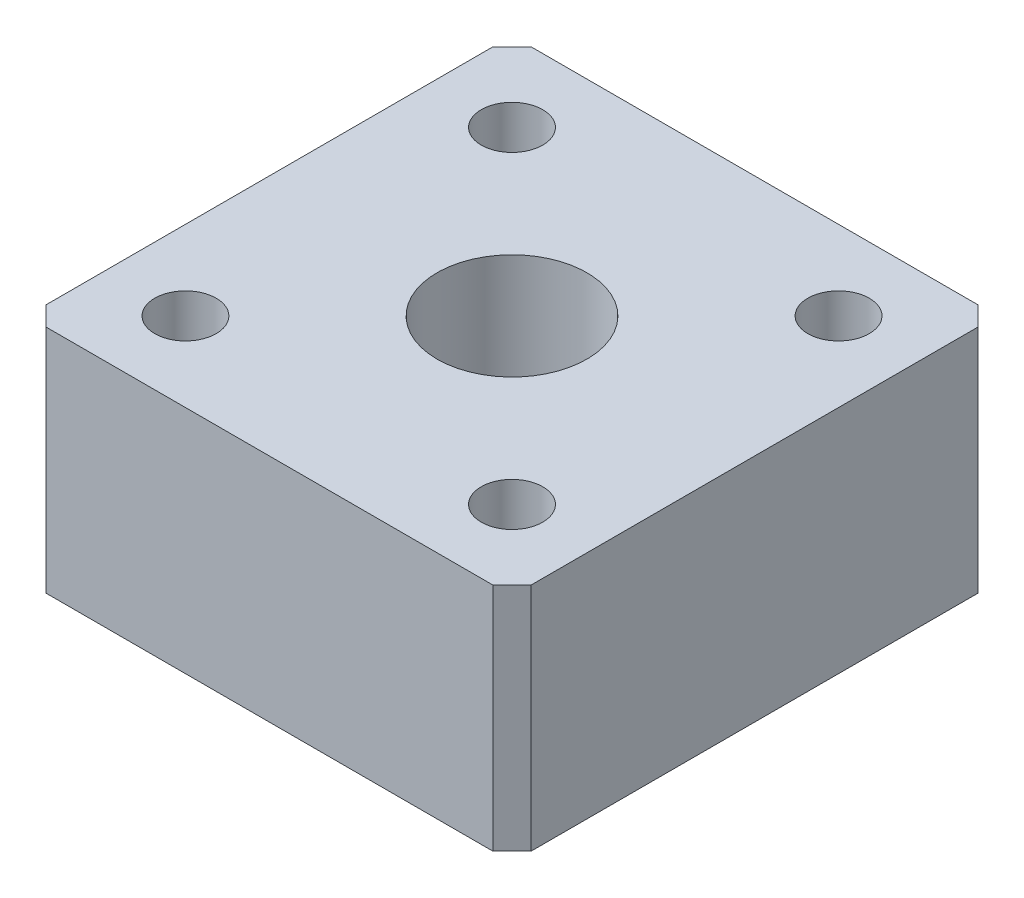
from build123d import *

# Parameters (mm, degrees)
SKETCH1_R             = 1.95
BOSS_EXTRUDE1_DEPTH   = 6
M2_TAPPED_HOLE2_D     = 1.6
M2_TAPPED_HOLE2_DEPTH = 6
M2_TAPPED_HOLE2_TIP   = 572.957422794


with BuildPart() as part:
    # Sketch1 → Boss-Extrude1 (new body)
    with BuildSketch(Plane(origin=(0, 0, 0), x_dir=(1, 0, 0), z_dir=(0, 1, 0))):
        Polygon((-6.315, 5.815), (-5.815, 6.315), (5.815, 6.315), (6.315, 5.815), (6.315, -5.815), (5.815, -6.315), (-5.815, -6.315), (-6.315, -5.815), align=None)
        with Locations(Location((0, 0, 0), (0, 0, 270))):
            Circle(SKETCH1_R, mode=Mode.SUBTRACT)
    extrude(amount=BOSS_EXTRUDE1_DEPTH)

    # M2 Tapped Hole2
    with Locations(Plane(origin=(0, 6, 0), x_dir=(-1, 0, 0), z_dir=(0, 1, 0))):
        with Locations((4.25, -4.25), (-4.25, -4.25), (-4.25, 4.25), (4.25, 4.25)):
            Hole(M2_TAPPED_HOLE2_D / 2, depth=M2_TAPPED_HOLE2_DEPTH)
            with Locations((0, 0, -(M2_TAPPED_HOLE2_DEPTH + M2_TAPPED_HOLE2_TIP / 2))):  # 0.16° drill point
                Cone(0, M2_TAPPED_HOLE2_D / 2, M2_TAPPED_HOLE2_TIP, mode=Mode.SUBTRACT)


solid = part.part
